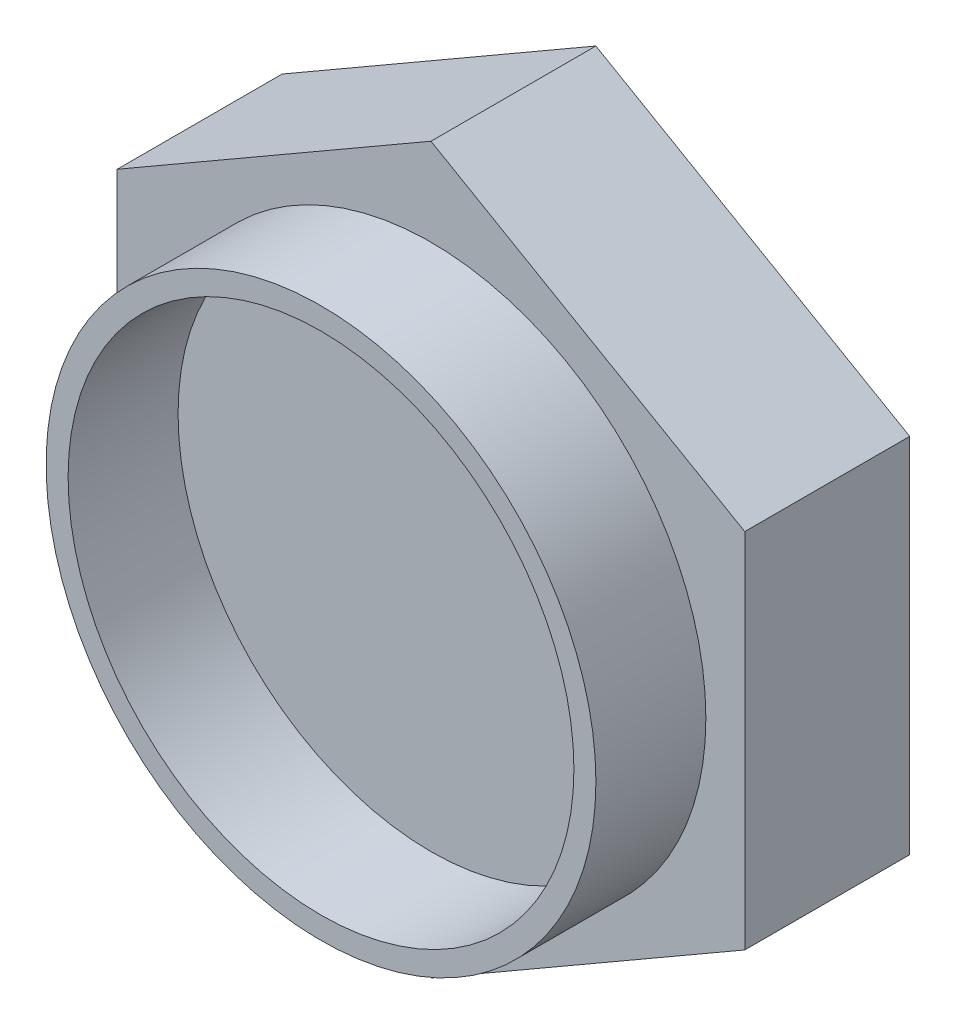
from build123d import *

# Parameters (mm, degrees)
SKETCH1_R           = 25
SKETCH1_R_2         = 23
BOSS_EXTRUDE1_DEPTH = 10
BOSS_EXTRUDE2_DEPTH = 15


with BuildPart() as part:
    # Sketch1 → Boss-Extrude1 (new body)
    with BuildSketch(Plane.XY):
        Circle(SKETCH1_R)
        Circle(SKETCH1_R_2, mode=Mode.SUBTRACT)
    extrude(amount=BOSS_EXTRUDE1_DEPTH)

    # Sketch2 → Boss-Extrude2 (add)
    with BuildSketch(Plane(origin=(0, 0, 0), x_dir=(-1, 0, 0), z_dir=(0, 0, -1))):
        Polygon((0, 32.951018806), (-28.536419367, 16.475509403), (-28.536419367, -16.475509403), (0, -32.951018806), (28.536419367, -16.475509403), (28.536419367, 16.475509403), align=None)
    extrude(amount=BOSS_EXTRUDE2_DEPTH)


solid = part.part
